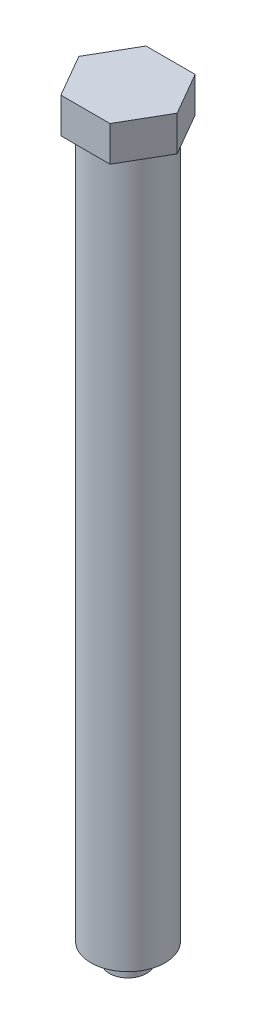
from build123d import *

# Parameters (mm, degrees)
SKETCH2_OUTSIDE_W  = 138.358
SKETCH2_OUTSIDE_H  = 138.358
CUT_EXTRUDE1_DEPTH = 32


with BuildPart() as part:
    # Sketch1 → Revolve1 (revolve)
    with BuildSketch(Plane.XY, mode=Mode.PRIVATE) as revolve1_sk:
        Polygon((0, 0), (10, 0), (10, 10), (20, 10), (20, 391), (26.5, 391), (26.5, 410), (0, 410), align=None)
    revolve(revolve1_sk.sketch.rotate(Axis((0, 0, 0), (0, 1, 0)), 90), axis=Axis((0, 0, 0), (0, 1, 0)))

    # Sketch2 outside → Cut-Extrude1 (cut)
    with BuildSketch(Plane(origin=(0, 410, 0), x_dir=(1, 0, 0), z_dir=(0, 1, 0))):
        Rectangle(SKETCH2_OUTSIDE_W, SKETCH2_OUTSIDE_H)
        Polygon((-26.5, 0), (-13.25, -22.9496732), (13.25, -22.9496732), (26.5, 0), (13.25, 22.9496732), (-13.25, 22.9496732), align=None, mode=Mode.SUBTRACT)
    extrude(amount=-CUT_EXTRUDE1_DEPTH, mode=Mode.SUBTRACT)


solid = part.part
